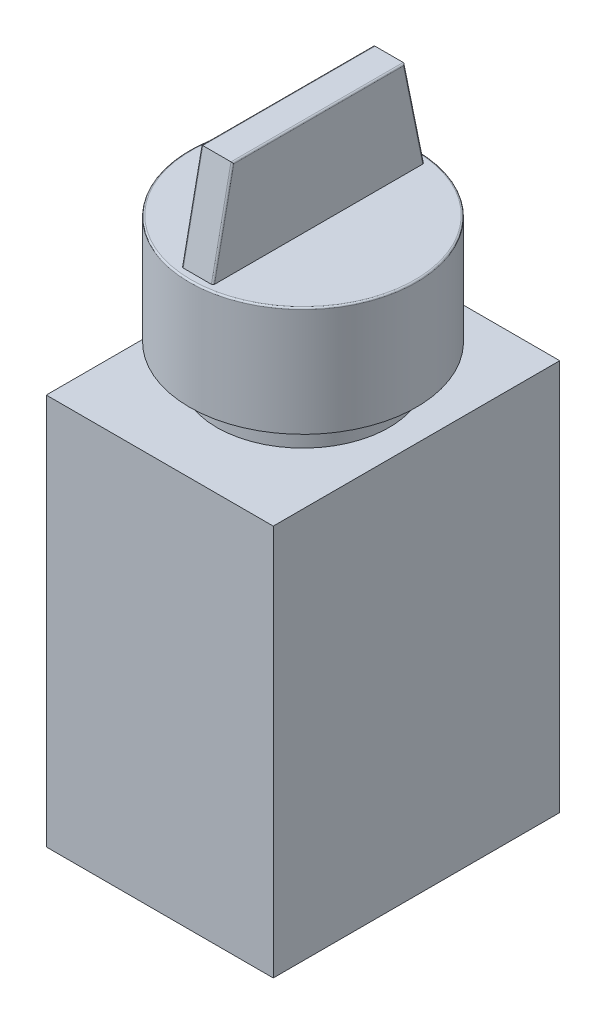
SolidWorks part; units mm, degrees
ref_plane "Front Plane" through (0, 0, 0) normal (0, 0, 1) x (1, 0, 0)
ref_plane "Top Plane" through (0, 0, 0) normal (0, 1, 0) x (1, 0, 0)
ref_plane "Right Plane" through (0, 0, 0) normal (1, 0, 0) x (0, 0, -1)
sketch "Sketch2" plane through (0, 0, 0) normal (0, 1, 0) x (1, 0, 0)
  circle A0 centre (0, 0) radius 14.5
  dimension "D1" = 29
extrude "Boss-Extrude1" add sketch "Sketch2" along normal blind 14
sketch "Sketch3" plane through (0, 14, 0) normal (0, 1, 0) x (1, 0, 0)
  line L1 (-2, -13.5) -> (2, -13.5)
  line L2 (-2, -13.5) -> (-2, 13.5)
  line L3 (-2, 13.5) -> (2, 13.5)
  line L4 (2, -13.5) -> (2, 13.5)
  line L5 (-2, -13.5) -> (2, 13.5) construction
  line L6 (-2, 13.5) -> (2, -13.5) construction
  point P0 (0, 0)
  dimension "D1" = 4
  dimension "D2" = 27
extrude "Boss-Extrude2" add sketch "Sketch3" along normal blind 12.3
sketch "Sketch4" plane through (2, 0, 0) normal (1, 0, 0) x (0, 0, -1)
  line L0 (0, 0) -> (0, 26.3) construction
  line L1 (-13.5, 26.3) -> (13.5, 26.3) construction
  line L2 (-13.5, 26.3) -> (-13.5, 14)
  line L3 (14.5, 14) -> (-14.5, 14) construction
  line L4 (-13.5, 26.3) -> (-13.5, 14) construction
  line L5 (-13.5, 14) -> (-11, 26.3)
  line L6 (-11, 26.3) -> (-13.5, 26.3)
  line L7 (11, 26.3) -> (13.5, 26.3)
  line L8 (13.5, 26.3) -> (13.5, 14)
  line L9 (13.5, 14) -> (11, 26.3)
  dimension "D1" = 22
extrude "Cut-Extrude1" cut sketch "Sketch4" against normal blind 12.3
sketch "Sketch5" plane through (0, 0, 0) normal (0, -1, 0) x (1, 0, 0)
  circle A0 centre (0, 0) radius 11
  dimension "D1" = 22
extrude "Boss-Extrude3" add sketch "Sketch5" along normal blind 4
sketch "Sketch6" plane through (0, -4, 0) normal (0, -1, 0) x (1, 0, 0)
  line L1 (-14.5, -18.3) -> (14.5, -18.3)
  line L2 (-14.5, -18.3) -> (-14.5, 18.3)
  line L3 (-14.5, 18.3) -> (14.5, 18.3)
  line L4 (14.5, -18.3) -> (14.5, 18.3)
  line L5 (-14.5, -18.3) -> (14.5, 18.3) construction
  line L6 (-14.5, 18.3) -> (14.5, -18.3) construction
  point P0 (0, 0)
  dimension "D1" = 29
  dimension "D2" = 36.6
extrude "Boss-Extrude4" add sketch "Sketch6" along normal blind 50
fillet "Fillet1" radius 0.2 7 edges at (0, 14, 14.5) (2, 20.15, 12.25) (2, 26.3, 0) (2, 20.15, -12.25) (-2, 26.3, 0) (-2, 20.15, 12.25) (-2, 20.15, -12.25)
